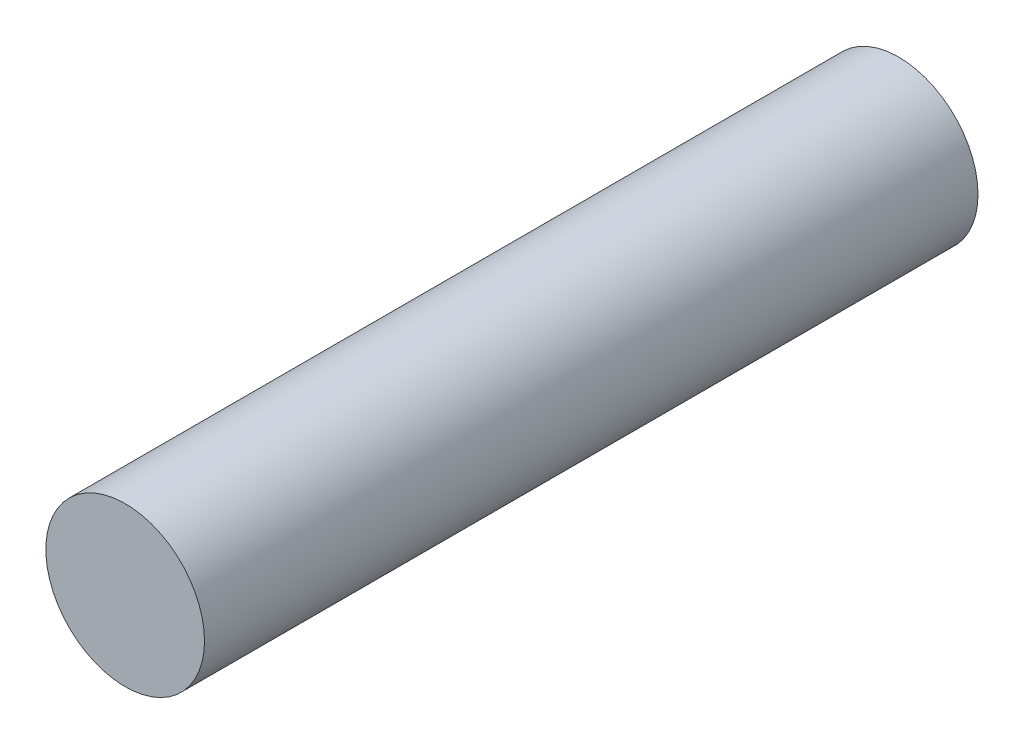
SolidWorks part; units mm, degrees
ref_plane "前视基准面" through (0, 0, 0) normal (0, 0, 1) x (1, 0, 0)
ref_plane "上视基准面" through (0, 0, 0) normal (0, 1, 0) x (1, 0, 0)
ref_plane "右视基准面" through (0, 0, 0) normal (1, 0, 0) x (0, 0, -1)
other "Configuration Table"
sketch "草图1" plane through (0, 0, 0) normal (0, 0, 1) x (1, 0, 0)
  circle A0 centre (0, 0) radius 4
  dimension "D1" = 8
extrude "凸台-拉伸1" add sketch "草图1" along normal blind 39
